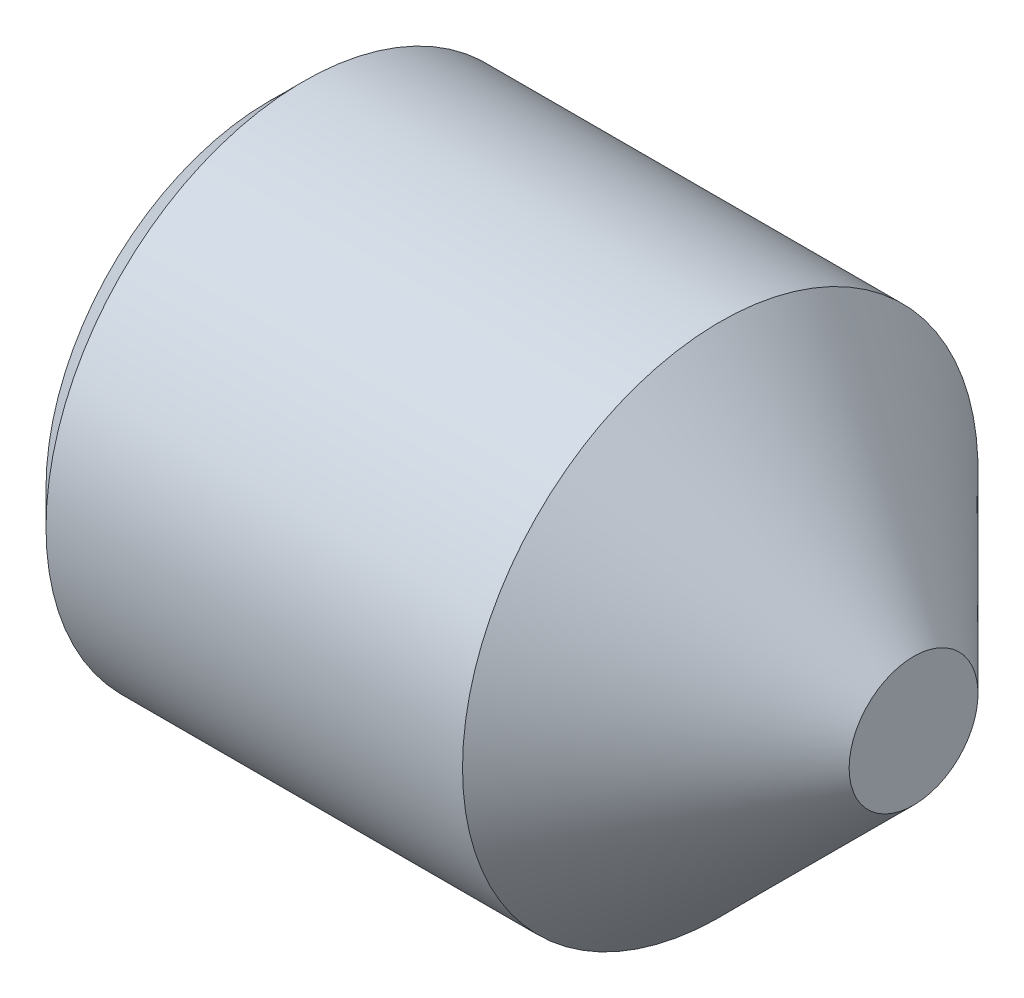
from build123d import *

# Parameters (mm, degrees)
CUT_EXTRUDE_1_DEPTH = 3


with BuildPart() as part:
    # 草图1 → Revolve 552 (revolve)
    with BuildSketch(Plane.XY, mode=Mode.PRIVATE) as revolve_552_sk:
        Polygon((0, 0), (10, 0), (10, 1), (7, 4), (0.536, 4), (0, 3.464), align=None)
    revolve(revolve_552_sk.sketch.rotate(Axis((-1.4104518, 0, 0), (1, 0, 0)), 90), axis=Axis((-1.4104518, 0, 0), (1, 0, 0)))

    # 草图2 → 切除-拉伸1 (cut)
    with BuildSketch(Plane.ZY):
        Polygon((2.29, 0), (1.145, 1.983198175), (-1.145, 1.983198175), (-2.29, 0), (-1.145, -1.983198175), (1.145, -1.983198175), align=None)
    extrude(amount=-CUT_EXTRUDE_1_DEPTH, mode=Mode.SUBTRACT)

    # 草图3 → 切除-旋转1 (revolve, cut)
    with BuildSketch(Plane.XY, mode=Mode.PRIVATE) as cut_revolve_1_sk:
        Polygon((3, 1.983198175), (4.145, 0), (3, 0), align=None)
    revolve(cut_revolve_1_sk.sketch.rotate(Axis((-0.121283255, 0, 0), (1, 0, 0)), 90), axis=Axis((-0.121283255, 0, 0), (1, 0, 0)), mode=Mode.SUBTRACT)


solid = part.part
